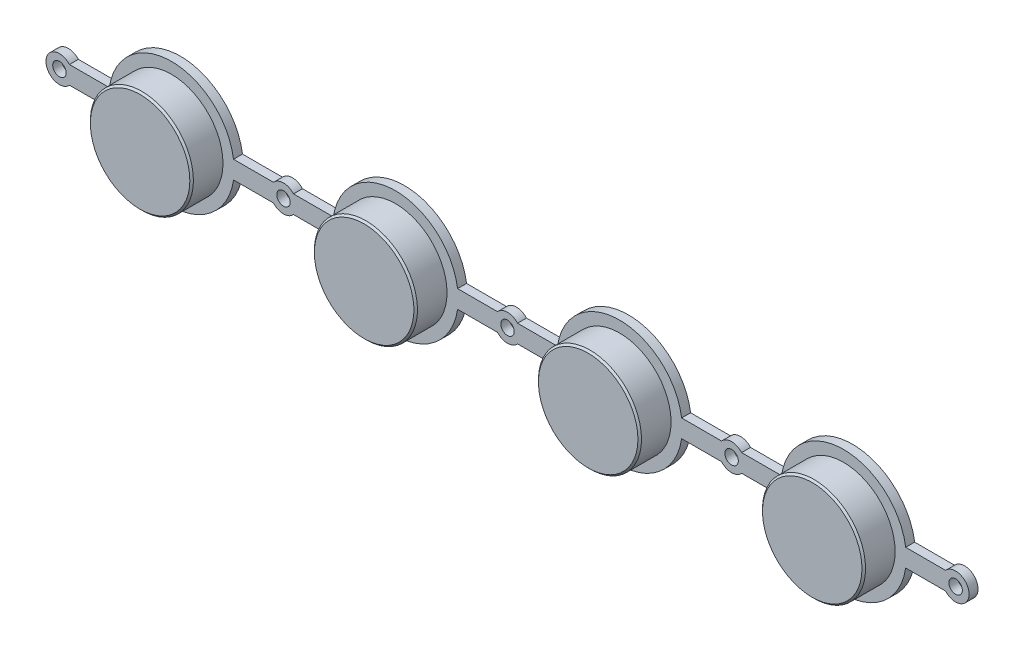
SolidWorks part; units mm, degrees
ref_plane "Front Plane" through (0, 0, 0) normal (0, 0, 1) x (1, 0, 0)
ref_plane "Top Plane" through (0, 0, 0) normal (0, 1, 0) x (1, 0, 0)
ref_plane "Right Plane" through (0, 0, 0) normal (1, 0, 0) x (0, 0, -1)
other "Configuration Table"
sketch "Sketch1" plane through (0, 0, 0) normal (0, 0, 1) x (1, 0, 0)
  line L0 (0, 0) -> (75, 0) construction
  line L1 (0, 0) -> (-12.5, 0) construction
  line L2 (75, 0) -> (87.5, 0) construction
  line L3 (-11.382, 1) -> (-6.9282, 1)
  line L4 (-11.382, -1) -> (-6.9282, -1)
  line L5 (6.9282, -1) -> (11.382, -1)
  line L6 (6.9282, 1) -> (11.382, 1)
  line L7 (13.618, 1) -> (18.0718, 1)
  line L8 (13.618, -1) -> (18.0718, -1)
  line L9 (31.9282, -1) -> (36.382, -1)
  line L10 (31.9282, 1) -> (36.382, 1)
  line L11 (38.618, 1) -> (43.0718, 1)
  line L12 (38.618, -1) -> (43.0718, -1)
  line L13 (56.9282, -1) -> (61.382, -1)
  line L14 (56.9282, 1) -> (61.382, 1)
  line L15 (63.618, 1) -> (68.0718, 1)
  line L16 (63.618, -1) -> (68.0718, -1)
  line L17 (81.9282, 1) -> (86.382, 1)
  line L18 (81.9282, -1) -> (86.382, -1)
  arc A4 (-6.9282, -1) -> (6.9282, -1) centre (0, 0) ccw
  arc A5 (18.0718, -1) -> (31.9282, -1) centre (25, 0) ccw
  arc A6 (43.0718, -1) -> (56.9282, -1) centre (50, 0) ccw
  arc A7 (68.0718, -1) -> (81.9282, -1) centre (75, 0) ccw
  circle A8 centre (12.5, 0) radius 0.75
  circle A9 centre (37.5, 0) radius 0.75
  circle A10 centre (62.5, 0) radius 0.75
  arc A11 (11.382, -1) -> (13.618, -1) centre (12.5, 0) ccw
  arc A12 (36.382, -1) -> (38.618, -1) centre (37.5, 0) ccw
  arc A13 (61.382, -1) -> (63.618, -1) centre (62.5, 0) ccw
  circle A14 centre (-12.5, 0) radius 0.75
  arc A15 (-11.382, 1) -> (-11.382, -1) centre (-12.5, 0) ccw
  circle A16 centre (87.5, 0) radius 0.75
  arc A17 (86.382, -1) -> (86.382, 1) centre (87.5, 0) ccw
  arc A18 (6.9282, 1) -> (-6.9282, 1) centre (0, 0) ccw
  arc A19 (13.618, 1) -> (11.382, 1) centre (12.5, 0) ccw
  arc A20 (31.9282, 1) -> (18.0718, 1) centre (25, 0) ccw
  arc A21 (38.618, 1) -> (36.382, 1) centre (37.5, 0) ccw
  arc A22 (56.9282, 1) -> (43.0718, 1) centre (50, 0) ccw
  arc A23 (63.618, 1) -> (61.382, 1) centre (62.5, 0) ccw
  arc A24 (81.9282, 1) -> (68.0718, 1) centre (75, 0) ccw
  dimension "D2" = 14
  dimension "D3" = 25
  dimension "D4" = 25
  dimension "D5" = 1.5
  dimension "D6" = 3
  dimension "D7" = 12.5
  dimension "D8" = 12.5
  dimension "D1" = 75
  dimension "D9" = 12.5
  dimension "D10" = 12.5
  dimension "D11" = 2
extrude "Boss-Extrude1" add sketch "Sketch1" along normal blind 1
sketch "Sketch2" plane through (0, 0, 1) normal (0, 0, 1) x (1, 0, 0)
  circle A0 centre (0, 0) radius 5.75
  circle A1 centre (25, 0) radius 5.75
  circle A2 centre (50, 0) radius 5.75
  circle A3 centre (75, 0) radius 5.75
  dimension "D1" = 11.5
extrude "Boss-Extrude2" add sketch "Sketch2" along normal blind 3.5
chamfer "Chamfer1" distance 0.2 angle 45 4 edges at (80.75, 0, 4.5) (55.75, 0, 4.5) (30.75, 0, 4.5) (5.75, 0, 4.5)
sketch "Sketch3" plane through (0, 0, 0) normal (0, 0, -1) x (-1, 0, 0)
  line L0 (-74.25, -0.75) -> (-74.25, -4)
  line L1 (-75.75, 4) -> (-74.25, 4)
  line L2 (-75.75, 4) -> (-75.75, 0.75)
  line L3 (-75.75, -4) -> (-74.25, -4)
  line L4 (-74.25, 4) -> (-74.25, 0.75)
  line L5 (-75.75, 4) -> (-74.25, -4) construction
  line L6 (-75.75, -4) -> (-74.25, 4) construction
  line L7 (-79, 0.75) -> (-75.75, 0.75)
  line L8 (-79, 0.75) -> (-79, -0.75)
  line L9 (-79, -0.75) -> (-75.75, -0.75)
  line L10 (-71, 0.75) -> (-71, -0.75)
  line L11 (-79, 0.75) -> (-71, -0.75) construction
  line L12 (-79, -0.75) -> (-71, 0.75) construction
  line L13 (-50.75, 4) -> (-49.25, 4)
  line L14 (-50.75, 4) -> (-50.75, 0.75)
  line L15 (-50.75, -4) -> (-49.25, -4)
  line L16 (-49.25, 4) -> (-49.25, 0.75)
  line L17 (-50.75, 4) -> (-49.25, -4) construction
  line L18 (-50.75, -4) -> (-49.25, 4) construction
  line L19 (-54, 0.75) -> (-50.75, 0.75)
  line L20 (-54, 0.75) -> (-54, -0.75)
  line L21 (-54, -0.75) -> (-50.75, -0.75)
  line L22 (-46, 0.75) -> (-46, -0.75)
  line L23 (-54, 0.75) -> (-46, -0.75) construction
  line L24 (-54, -0.75) -> (-46, 0.75) construction
  line L25 (-29, 0.75) -> (-25.75, 0.75)
  line L26 (-29, 0.75) -> (-29, -0.75)
  line L27 (-29, -0.75) -> (-25.75, -0.75)
  line L28 (-21, 0.75) -> (-21, -0.75)
  line L29 (-29, 0.75) -> (-21, -0.75) construction
  line L30 (-29, -0.75) -> (-21, 0.75) construction
  line L31 (-25.75, 4) -> (-24.25, 4)
  line L32 (-25.75, 4) -> (-25.75, 0.75)
  line L33 (-25.75, -4) -> (-24.25, -4)
  line L34 (-24.25, 4) -> (-24.25, 0.75)
  line L35 (-25.75, 4) -> (-24.25, -4) construction
  line L36 (-25.75, -4) -> (-24.25, 4) construction
  line L37 (-4, 0.75) -> (-0.75, 0.75)
  line L38 (-4, 0.75) -> (-4, -0.75)
  line L39 (-4, -0.75) -> (-0.75, -0.75)
  line L40 (4, 0.75) -> (4, -0.75)
  line L41 (-4, 0.75) -> (4, -0.75) construction
  line L42 (-4, -0.75) -> (4, 0.75) construction
  line L43 (-0.75, 4) -> (0.75, 4)
  line L44 (-0.75, 4) -> (-0.75, 0.75)
  line L45 (-0.75, -4) -> (0.75, -4)
  line L46 (0.75, 4) -> (0.75, 0.75)
  line L47 (-0.75, 4) -> (0.75, -4) construction
  line L48 (-0.75, -4) -> (0.75, 4) construction
  line L49 (-74.25, -0.75) -> (-71, -0.75)
  line L51 (-75.75, -0.75) -> (-75.75, -4)
  line L54 (-74.25, 0.75) -> (-71, 0.75)
  line L58 (-49.25, 0.75) -> (-46, 0.75)
  line L60 (-49.25, -0.75) -> (-49.25, -4)
  line L61 (-49.25, -0.75) -> (-46, -0.75)
  line L63 (-50.75, -0.75) -> (-50.75, -4)
  line L65 (-25.75, -0.75) -> (-25.75, -4)
  line L68 (-24.25, 0.75) -> (-21, 0.75)
  line L70 (-24.25, -0.75) -> (-24.25, -4)
  line L71 (-24.25, -0.75) -> (-21, -0.75)
  line L73 (0.75, 0.75) -> (4, 0.75)
  line L76 (-0.75, -0.75) -> (-0.75, -4)
  line L78 (0.75, -0.75) -> (0.75, -4)
  line L79 (0.75, -0.75) -> (4, -0.75)
  point P0 (-75, 0)
  point P6 (-75, 0)
  point P11 (-50, 0)
  point P17 (-50, 0)
  point P22 (-25, 0)
  point P28 (-25, 0)
  point P33 (0, 0)
  point P39 (0, 0)
  dimension "D1" = 8
  dimension "D2" = 8
  dimension "D3" = 1.5
  dimension "D4" = 1.5
  dimension "D5" = 8
  dimension "D6" = 8
  dimension "D7" = 1.5
  dimension "D8" = 1.5
  dimension "D9" = 8
  dimension "D10" = 8
  dimension "D11" = 1.5
  dimension "D12" = 1.5
  dimension "D13" = 8
  dimension "D14" = 8
  dimension "D15" = 1.5
  dimension "D16" = 1.5
extrude "Boss-Extrude3" add sketch "Sketch3" along normal blind 2
chamfer "Chamfer2" distance 1.6 angle 45 16 edges at (-4, 0, -2) (0, -4, -2) (0, 4, -2) (4, 0, -2) (25, 4, -2) (21, 0, -2) (29, 0, -2) (25, -4, -2) (50, 4, -2) (46, 0, -2) (50, -4, -2) (54, 0, -2) (75, 4, -2) (79, 0, -2) (71, 0, -2) (75, -4, -2)
